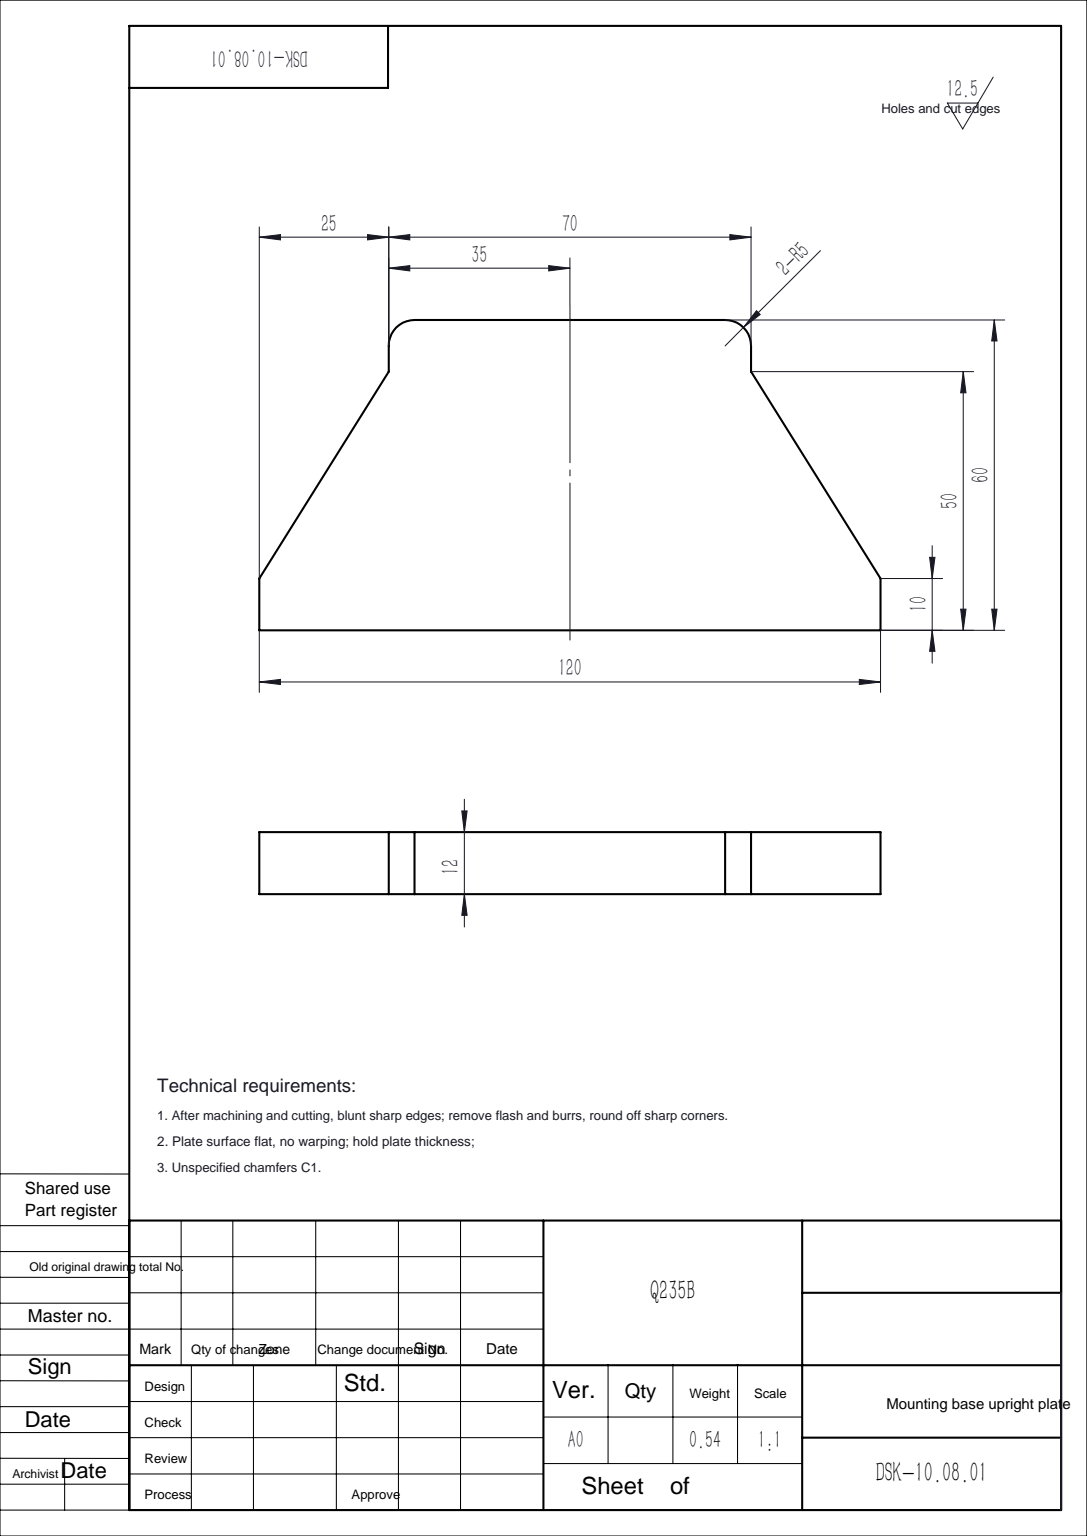
from build123d import *

# Parameters (mm, degrees)
BOSS_EXTRUDE1_DEPTH = 6
FILLET1_R           = 5


with BuildPart() as part:
    # Sketch1 → Boss-Extrude1 (new, symmetric)
    with BuildSketch(Plane.XY):
        Polygon((-60, 0), (60, 0), (60, 10), (35, 50), (35, 60), (-35, 60), (-35, 50), (-60, 10), align=None)
    extrude(amount=BOSS_EXTRUDE1_DEPTH, both=True)

    # Fillet1
    fillet1_edges = [part.edges().sort_by_distance(p)[0] for p in [
        (-35, 60, 0),
        (35, 60, 0),
    ]]
    fillet(fillet1_edges, radius=FILLET1_R)


solid = part.part
